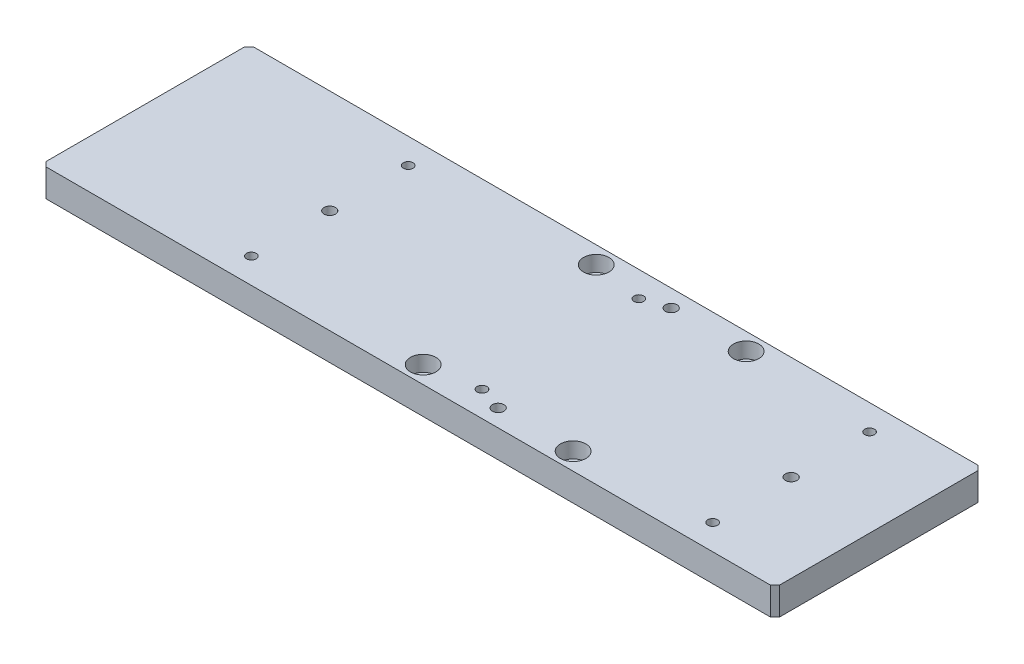
from build123d import *

# Parameters (mm, degrees)
SKETCH_1_W                   = 318
SKETCH_1_H                   = 90
EXTRUDE_1_DEPTH              = 12
HOLE_WIZARD_M6_1_D           = 6.6
HOLE_WIZARD_M6_1_CBORE_D     = 11
HOLE_WIZARD_M6_1_CBORE_DEPTH = 6.8
HOLE_WIZARD_M5_1_D           = 4.2
F_5_0MM_1_D                  = 5
F_5_0MM_1_DEPTH              = 6
F_5_0MM_1_TIP                = 1.502151548
F_5_0MM_2_D                  = 5
F_5_0MM_2_DEPTH              = 5
F_5_0MM_2_TIP                = 1.502151548
CHAMFER_1_SIZE               = 2


with BuildPart() as part:
    # 草图1 → 凸台-拉伸1 (new body)
    with BuildSketch(Plane(origin=(0, 0, 0), x_dir=(1, 0, 0), z_dir=(0, 1, 0))):
        Rectangle(SKETCH_1_W, SKETCH_1_H)
    extrude(amount=EXTRUDE_1_DEPTH)

    # M6 六角圆柱头螺钉的柱形沉头孔1 (through all)
    with Locations(Plane(origin=(0, 12, 0), x_dir=(1, 0, 0), z_dir=(0, 1, 0))):
        with Locations((64, 37.5), (-1, 37.5), (-1, -37.5), (64, -37.5)):
            CounterBoreHole(HOLE_WIZARD_M6_1_D / 2, HOLE_WIZARD_M6_1_CBORE_D / 2, HOLE_WIZARD_M6_1_CBORE_DEPTH)

    # M5 螺纹孔1 (through all)
    with Locations(Plane(origin=(0, 12, 0), x_dir=(1, 0, 0), z_dir=(0, 1, 0))):
        with Locations((121, 34), (121, -34), (21, 34), (21, -34), (-79, 34), (-79, -34)):
            Hole(HOLE_WIZARD_M5_1_D / 2)

    # Ø5.0mm 暗销孔1
    with Locations(Plane(origin=(0, 12, 0), x_dir=(1, 0, 0), z_dir=(0, 1, 0))):
        with Locations((121, 0), (-79, 0)):
            Hole(F_5_0MM_1_D / 2, depth=F_5_0MM_1_DEPTH)
            with Locations((0, 0, -(F_5_0MM_1_DEPTH + F_5_0MM_1_TIP / 2))):  # 118° drill point
                Cone(0, F_5_0MM_1_D / 2, F_5_0MM_1_TIP, mode=Mode.SUBTRACT)

    # Ø5.0mm 暗销孔2
    with Locations(Plane(origin=(0, 12, 0), x_dir=(1, 0, 0), z_dir=(0, 1, 0))):
        with Locations((31.5, -37.5), (31.5, 37.5)):
            Hole(F_5_0MM_2_D / 2, depth=F_5_0MM_2_DEPTH)
            with Locations((0, 0, -(F_5_0MM_2_DEPTH + F_5_0MM_2_TIP / 2))):  # 118° drill point
                Cone(0, F_5_0MM_2_D / 2, F_5_0MM_2_TIP, mode=Mode.SUBTRACT)

    # 倒角1
    chamfer_1_edges = [part.edges().sort_by_distance(p)[0] for p in [
        (159, 6, 45),
        (-159, 6, 45),
        (-159, 6, -45),
        (159, 6, -45),
    ]]
    chamfer(chamfer_1_edges, length=CHAMFER_1_SIZE)


solid = part.part
